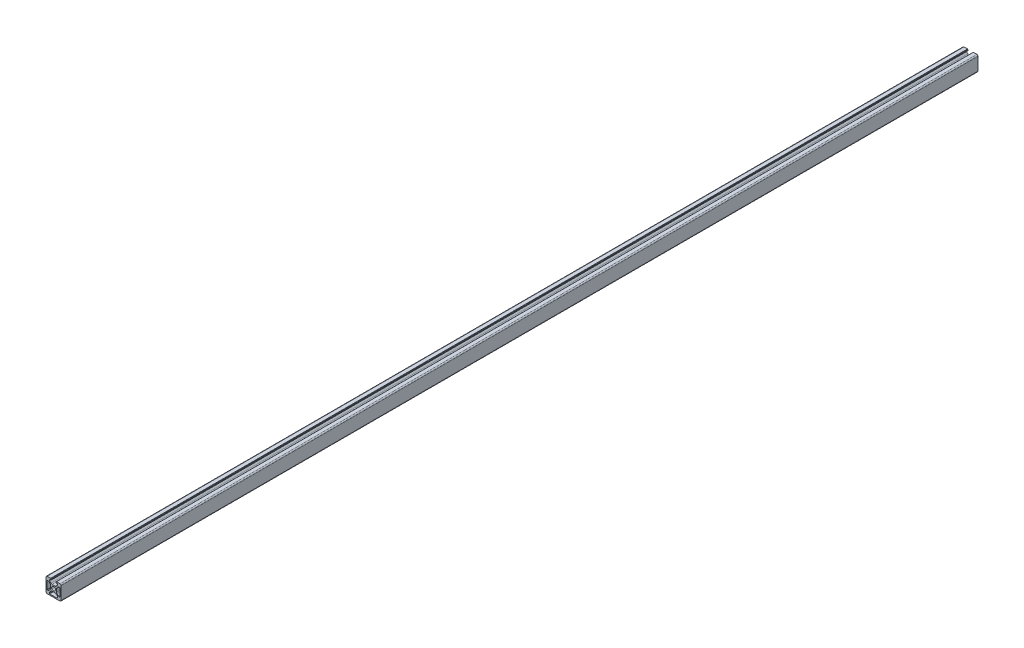
from build123d import *

# Parameters (mm, degrees)
SKETCH_1_R      = 2.5
EXTRUDE_1_DEPTH = 1215


with BuildPart() as part:
    # 草图1 → 凸台-拉伸1 (new body)
    with BuildSketch(Plane.XY):
        with BuildLine():
            Line((1573.123527995, 1294.902726123), (1571.136522226, 1296.889731891))
            ThreePointArc((1571.136522226, 1296.889731891), (1571.071490401, 1296.987058896), (1571.048654261, 1297.101863926))
            Line((1571.048654261, 1297.101863926), (1571.048654261, 1298.316939685))
            ThreePointArc((1571.048654261, 1298.316939685), (1571.136522226, 1298.52907172), (1571.348654261, 1298.616939685))
            Line((1571.348654261, 1298.616939685), (1573.148654261, 1298.616939685))
            ThreePointArc((1573.148654261, 1298.616939685), (1573.360786295, 1298.704807651), (1573.448654261, 1298.916939685))
            Line((1573.448654261, 1298.916939685), (1573.448654261, 1299.616939685))
            ThreePointArc((1573.448654261, 1299.616939685), (1573.360786295, 1299.82907172), (1573.148654261, 1299.916939685))
            Line((1573.148654261, 1299.916939685), (1572.948654261, 1299.916939685))
            Line((1572.948654261, 1299.916939685), (1572.948654261, 1300.116939685))
            ThreePointArc((1572.948654261, 1300.116939685), (1572.860786295, 1300.32907172), (1572.648654261, 1300.416939685))
            Line((1572.648654261, 1300.416939685), (1568.048654261, 1300.416939685))
            ThreePointArc((1568.048654261, 1300.416939685), (1566.987994089, 1299.977599857), (1566.548654261, 1298.916939685))
            Line((1566.548654261, 1298.916939685), (1566.548654261, 1281.916939685))
            ThreePointArc((1566.548654261, 1281.916939685), (1566.987994089, 1280.856279514), (1568.048654261, 1280.416939685))
            Line((1568.048654261, 1280.416939685), (1585.048654261, 1280.416939685))
            ThreePointArc((1585.048654261, 1280.416939685), (1586.109314432, 1280.856279514), (1586.548654261, 1281.916939685))
            Line((1586.548654261, 1281.916939685), (1586.548654261, 1298.916939685))
            ThreePointArc((1586.548654261, 1298.916939685), (1586.109314432, 1299.977599857), (1585.048654261, 1300.416939685))
            Line((1585.048654261, 1300.416939685), (1580.448654261, 1300.416939685))
            ThreePointArc((1580.448654261, 1300.416939685), (1580.236522226, 1300.32907172), (1580.148654261, 1300.116939685))
            Line((1580.148654261, 1300.116939685), (1580.148654261, 1299.916939685))
            Line((1580.148654261, 1299.916939685), (1579.948654261, 1299.916939685))
            ThreePointArc((1579.948654261, 1299.916939685), (1579.736522226, 1299.82907172), (1579.648654261, 1299.616939685))
            Line((1579.648654261, 1299.616939685), (1579.648654261, 1298.916939685))
            ThreePointArc((1579.648654261, 1298.916939685), (1579.736522226, 1298.704807651), (1579.94865426, 1298.616939685))
            Line((1579.94865426, 1298.616939685), (1581.748654261, 1298.616939685))
            ThreePointArc((1581.748654261, 1298.616939685), (1581.960786295, 1298.52907172), (1582.048654261, 1298.316939685))
            Line((1582.048654261, 1298.316939685), (1582.048654261, 1297.101863926))
            ThreePointArc((1582.048654261, 1297.101863926), (1582.02581812, 1296.987058896), (1581.960786295, 1296.889731891))
            Line((1581.960786295, 1296.889731891), (1579.973780526, 1294.902726123))
            ThreePointArc((1579.973780526, 1294.902726123), (1579.324933829, 1294.46918062), (1578.559566964, 1294.316939685))
            Line((1578.559566964, 1294.316939685), (1574.537741557, 1294.316939685))
            ThreePointArc((1574.537741557, 1294.316939685), (1573.772374693, 1294.46918062), (1573.123527995, 1294.902726123))
        make_face()
        with Locations((1576.548654261, 1290.416939685)):
            Circle(SKETCH_1_R, mode=Mode.SUBTRACT)
        with BuildLine():
            Line((1572.648654261, 1292.427852389), (1572.648654261, 1288.406026982))
            ThreePointArc((1572.648654261, 1288.406026982), (1572.496413326, 1287.640660117), (1572.062867823, 1286.99181342))
            Line((1572.062867823, 1286.99181342), (1569.987994089, 1284.916939685))
            Line((1569.987994089, 1284.916939685), (1568.348654261, 1284.916939685))
            ThreePointArc((1568.348654261, 1284.916939685), (1568.136522226, 1285.004807651), (1568.048654261, 1285.216939685))
            Line((1568.048654261, 1285.216939685), (1568.048654261, 1295.616939685))
            ThreePointArc((1568.048654261, 1295.616939685), (1568.136522226, 1295.82907172), (1568.348654261, 1295.916939685))
            Line((1568.348654261, 1295.916939685), (1569.86373002, 1295.916939685))
            ThreePointArc((1569.86373002, 1295.916939685), (1569.97853505, 1295.894103545), (1570.075862055, 1295.82907172))
            Line((1570.075862055, 1295.82907172), (1572.062867823, 1293.842065951))
            ThreePointArc((1572.062867823, 1293.842065951), (1572.496413326, 1293.193219254), (1572.648654261, 1292.427852389))
        make_face(mode=Mode.SUBTRACT)
        with BuildLine():
            Line((1581.034440698, 1293.842065951), (1583.021446467, 1295.82907172))
            ThreePointArc((1583.021446467, 1295.82907172), (1583.118773471, 1295.894103545), (1583.233578501, 1295.916939685))
            Line((1583.233578501, 1295.916939685), (1584.748654261, 1295.916939685))
            ThreePointArc((1584.748654261, 1295.916939685), (1584.960786295, 1295.82907172), (1585.048654261, 1295.616939685))
            Line((1585.048654261, 1295.616939685), (1585.048654261, 1285.216939685))
            ThreePointArc((1585.048654261, 1285.216939685), (1584.960786295, 1285.004807651), (1584.748654261, 1284.916939685))
            Line((1584.748654261, 1284.916939685), (1583.109314432, 1284.916939685))
            Line((1583.109314432, 1284.916939685), (1581.034440698, 1286.99181342))
            ThreePointArc((1581.034440698, 1286.99181342), (1580.600895196, 1287.640660117), (1580.448654261, 1288.406026982))
            Line((1580.448654261, 1288.406026982), (1580.448654261, 1292.427852389))
            ThreePointArc((1580.448654261, 1292.427852389), (1580.600895196, 1293.193219254), (1581.034440698, 1293.842065951))
        make_face(mode=Mode.SUBTRACT)
        with BuildLine():
            Line((1574.537741557, 1286.516939685), (1578.559566964, 1286.516939685))
            ThreePointArc((1578.559566964, 1286.516939685), (1579.324933829, 1286.36469875), (1579.973780526, 1285.931153248))
            Line((1579.973780526, 1285.931153248), (1581.960786295, 1283.944147479))
            ThreePointArc((1581.960786295, 1283.944147479), (1582.02581812, 1283.846820475), (1582.048654261, 1283.732015445))
            Line((1582.048654261, 1283.732015445), (1582.048654261, 1282.216939685))
            ThreePointArc((1582.048654261, 1282.216939685), (1581.960786295, 1282.004807651), (1581.748654261, 1281.916939685))
            Line((1581.748654261, 1281.916939685), (1571.348654261, 1281.916939685))
            ThreePointArc((1571.348654261, 1281.916939685), (1571.136522226, 1282.004807651), (1571.048654261, 1282.216939685))
            Line((1571.048654261, 1282.216939685), (1571.048654261, 1283.732015445))
            ThreePointArc((1571.048654261, 1283.732015445), (1571.071490401, 1283.846820475), (1571.136522226, 1283.944147479))
            Line((1571.136522226, 1283.944147479), (1573.123527995, 1285.931153248))
            ThreePointArc((1573.123527995, 1285.931153248), (1573.772374693, 1286.36469875), (1574.537741557, 1286.516939685))
        make_face(mode=Mode.SUBTRACT)
    extrude(amount=EXTRUDE_1_DEPTH)


solid = part.part
